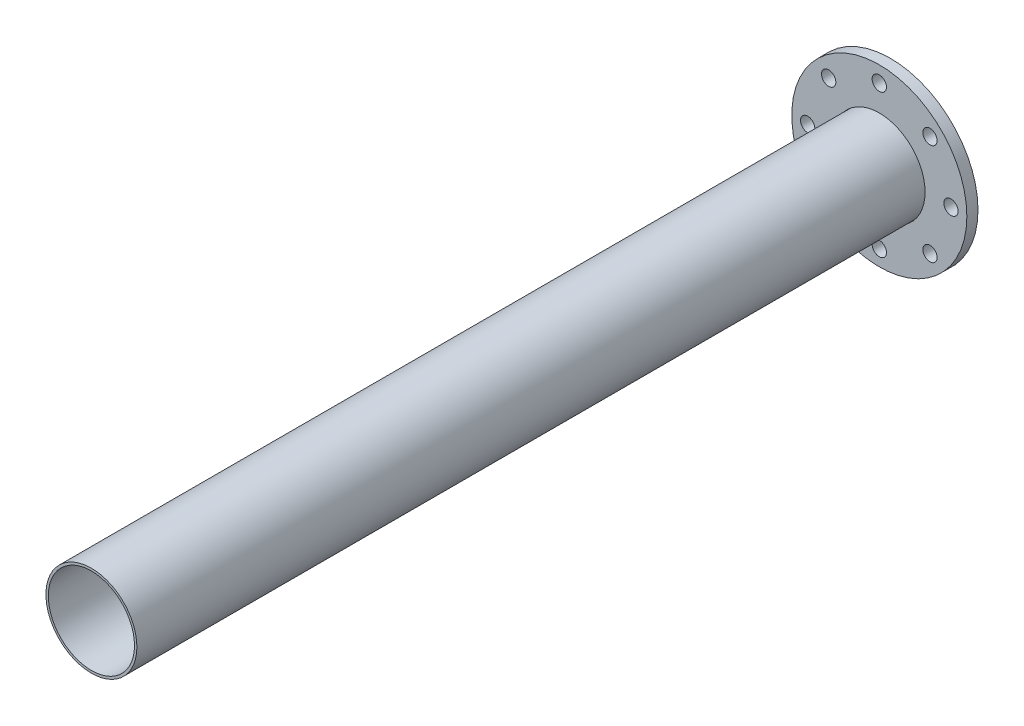
from build123d import *

# Parameters (mm, degrees)
SKETCH1_R           = 110
SKETCH1_R_2         = 57.5
SKETCH1_R_3         = 9
BOSS_EXTRUDE1_DEPTH = 14
SKETCH2_R           = 57.15
SKETCH2_R_2         = 54.15
BOSS_EXTRUDE2_DEPTH = 1000


with BuildPart() as part:
    # Sketch1 → Boss-Extrude1 (new body)
    with BuildSketch(Plane.XY):
        Circle(SKETCH1_R)
        Circle(SKETCH1_R_2, mode=Mode.SUBTRACT)
        with Locations((0, 90)):
            Circle(SKETCH1_R_3, mode=Mode.SUBTRACT)
        with Locations((63.639610307, 63.639610307)):
            Circle(SKETCH1_R_3, mode=Mode.SUBTRACT)
        with Locations((90, 0)):
            Circle(SKETCH1_R_3, mode=Mode.SUBTRACT)
        with Locations((63.639610307, -63.639610307)):
            Circle(SKETCH1_R_3, mode=Mode.SUBTRACT)
        with Locations((0, -90)):
            Circle(SKETCH1_R_3, mode=Mode.SUBTRACT)
        with Locations((-63.639610307, -63.639610307)):
            Circle(SKETCH1_R_3, mode=Mode.SUBTRACT)
        with Locations((-90, 0)):
            Circle(SKETCH1_R_3, mode=Mode.SUBTRACT)
        with Locations((-63.639610307, 63.639610307)):
            Circle(SKETCH1_R_3, mode=Mode.SUBTRACT)
    extrude(amount=BOSS_EXTRUDE1_DEPTH)


with BuildPart() as body_2:
    # Sketch2 → Boss-Extrude2 (new body)
    with BuildSketch(Plane.XY.offset(4)):
        Circle(SKETCH2_R)
        Circle(SKETCH2_R_2, mode=Mode.SUBTRACT)
    extrude(amount=BOSS_EXTRUDE2_DEPTH)


solid = Compound([part.part, body_2.part])
